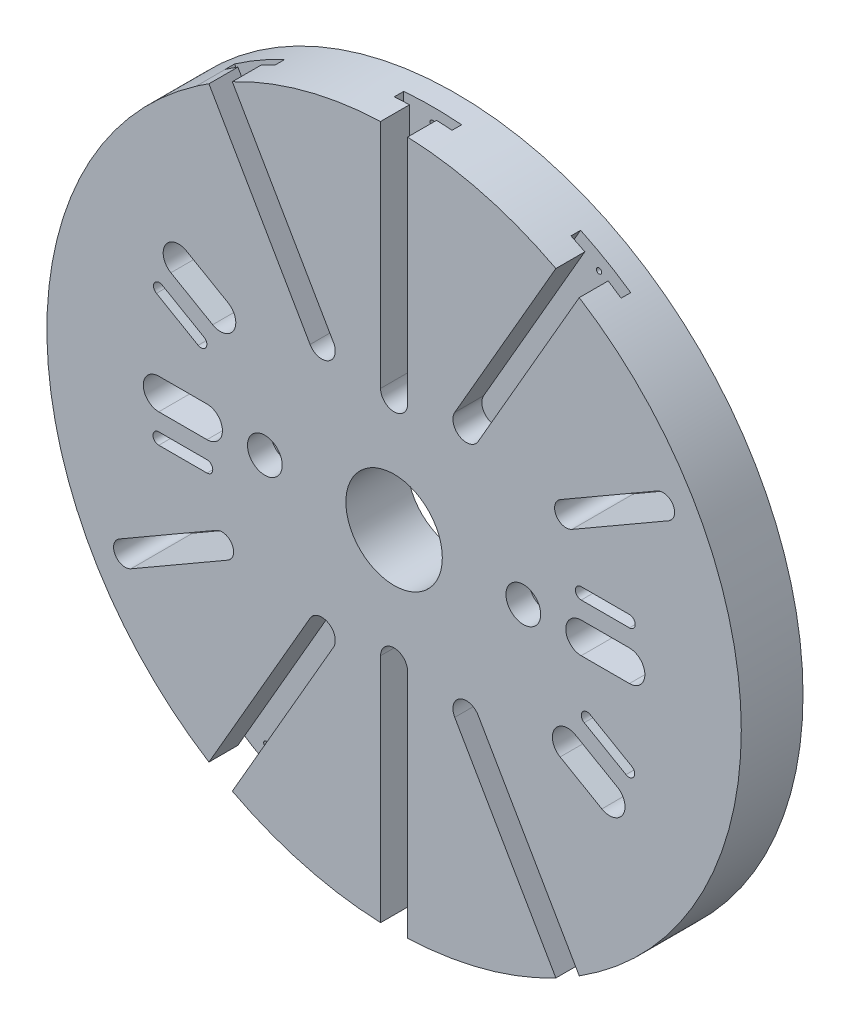
from build123d import *

# Parameters (mm, degrees)
SKETCH1_R           = 180
SKETCH1_R_2         = 25
BOSS_EXTRUDE1_DEPTH = 32
SKETCH2_R           = 5.5
CUT_EXTRUDE1_DEPTH  = 257.561883373
CUT_EXTRUDE3_DEPTH  = 257.561883373
CUT_EXTRUDE4_DEPTH  = 5
CUT_EXTRUDE5_REACH  = 258.562
SKETCH7_R           = 1.375
CUT_EXTRUDE6_DEPTH  = 257.561883373
CUT_EXTRUDE7_DEPTH  = 17.2
CUT_EXTRUDE8_START  = -32
CUT_EXTRUDE8_DEPTH  = 15
SKETCH11_R          = 9
CUT_EXTRUDE9_DEPTH  = 12
SKETCH12_R          = 5.5
CUT_EXTRUDE10_DEPTH = 11


with BuildPart() as part:
    # Sketch1 → Boss-Extrude1 (new body)
    with BuildSketch(Plane.XY):
        Circle(SKETCH1_R)
        Circle(SKETCH1_R_2, mode=Mode.SUBTRACT)
    extrude(amount=BOSS_EXTRUDE1_DEPTH)

    # Sketch2 → Cut-Extrude1 (cut, through all)
    with BuildSketch(Plane.XY.offset(32)):
        with Locations((67, 0)):
            Circle(SKETCH2_R)
        with Locations(Location((-67, 0, 0), (0, 0, 180))):
            Circle(SKETCH2_R)
    extrude(amount=-CUT_EXTRUDE1_DEPTH, mode=Mode.SUBTRACT)

    # Sketch3 → Cut-Extrude3 (cut, through all)
    with BuildSketch(Plane.XY.offset(32)):
        with BuildLine():
            Line((-86.20061659, -56.696152423), (-136.430090009, -85.696152423))
            ThreePointArc((-136.430090009, -85.696152423), (-144.626242432, -83.5), (-142.430090009, -75.303847577))
            Line((-142.430090009, -75.303847577), (-92.20061659, -46.303847577))
            ThreePointArc((-92.20061659, -46.303847577), (-84.004464167, -48.5), (-86.20061659, -56.696152423))
        make_face()
        with BuildLine():
            Line((86.20061659, 56.696152423), (136.430090009, 85.696152423))
            ThreePointArc((136.430090009, 85.696152423), (144.626242432, 83.5), (142.430090009, 75.303847577))
            Line((142.430090009, 75.303847577), (92.20061659, 46.303847577))
            ThreePointArc((92.20061659, 46.303847577), (84.004464167, 48.5), (86.20061659, 56.696152423))
        make_face()
    extrude(amount=-CUT_EXTRUDE3_DEPTH, mode=Mode.SUBTRACT)

    # Sketch5 → Cut-Extrude4 (cut)
    with BuildSketch(Plane(origin=(0, 0, 12), x_dir=(-1, 0, 0), z_dir=(0, 0, -1))):
        with BuildLine():
            Line((15, 60), (15, 264.061054266))
            Line((15, 264.061054266), (-15, 249.37568409))
            Line((-15, 249.37568409), (-15, 60))
            ThreePointArc((-15, 60), (0, 45), (15, 60))
        make_face()
        with BuildLine():
            Line((-91.956389003, 189.273137833), (-117.937151116, 174.273137833))
            Line((-117.937151116, 174.273137833), (-50.490381057, 57.451905284))
            ThreePointArc((-50.490381057, 57.451905284), (-30, 51.961524227), (-24.509618943, 72.451905284))
            Line((-24.509618943, 72.451905284), (-91.956389003, 189.273137833))
        make_face()
        with BuildLine():
            Line((91.956389003, 189.273137833), (24.509618943, 72.451905284))
            ThreePointArc((24.509618943, 72.451905284), (30, 51.961524227), (50.490381057, 57.451905284))
            Line((50.490381057, 57.451905284), (117.937151116, 174.273137833))
            Line((117.937151116, 174.273137833), (91.956389003, 189.273137833))
        make_face()
        with BuildLine():
            Line((91.956389003, -189.273137833), (117.937151116, -174.273137833))
            Line((117.937151116, -174.273137833), (50.490381057, -57.451905284))
            ThreePointArc((50.490381057, -57.451905284), (30, -51.961524227), (24.509618943, -72.451905284))
            Line((24.509618943, -72.451905284), (91.956389003, -189.273137833))
        make_face()
        with BuildLine():
            Line((-91.956389003, -189.273137833), (-24.509618943, -72.451905284))
            ThreePointArc((-24.509618943, -72.451905284), (-30, -51.961524227), (-50.490381057, -57.451905284))
            Line((-50.490381057, -57.451905284), (-117.937151116, -174.273137833))
            Line((-117.937151116, -174.273137833), (-91.956389003, -189.273137833))
        make_face()
        with BuildLine():
            Line((10, -264.061054266), (-15, -249.37568409))
            Line((-15, -249.37568409), (-15, -60))
            ThreePointArc((-15, -60), (0, -45), (15, -60))
            Line((15, -60), (10, -264.061054266))
        make_face()
    extrude(amount=-CUT_EXTRUDE4_DEPTH, mode=Mode.SUBTRACT)

    # Sketch6 → Cut-Extrude5 (cut, up to next)
    with BuildSketch(Plane.XY.offset(32), mode=Mode.PRIVATE) as cut_extrude5_sk1:
        with BuildLine():
            Line((-95.884592233, -180.076985411), (-108.008947886, -173.076985411))
            Line((-108.008947886, -173.076985411), (-43.562177826, -61.451905284))
            ThreePointArc((-43.562177826, -61.451905284), (-34, -58.889727457), (-31.437822174, -68.451905284))
            Line((-31.437822174, -68.451905284), (-95.884592233, -180.076985411))
        make_face()
    cut_extrude5_tool1 = extrude(cut_extrude5_sk1.sketch, amount=-CUT_EXTRUDE5_REACH, mode=Mode.PRIVATE) & part.part
    # Sketch6 → Cut-Extrude5 (cut, up to next)
    with BuildSketch(Plane.XY.offset(32), mode=Mode.PRIVATE) as cut_extrude5_sk2:
        with BuildLine():
            Line((-7, -254.443680545), (-7, -60))
            ThreePointArc((-7, -60), (0, -53), (7, -60))
            Line((7, -60), (7, -245.63245844))
            Line((7, -245.63245844), (-7, -254.443680545))
        make_face()
    cut_extrude5_tool2 = extrude(cut_extrude5_sk2.sketch, amount=-CUT_EXTRUDE5_REACH, mode=Mode.PRIVATE) & part.part
    # Sketch6 → Cut-Extrude5 (cut, up to next)
    with BuildSketch(Plane.XY.offset(32), mode=Mode.PRIVATE) as cut_extrude5_sk3:
        with BuildLine():
            Line((43.562177826, -61.451905284), (108.008947886, -173.076985411))
            Line((108.008947886, -173.076985411), (95.884592233, -180.076985411))
            Line((95.884592233, -180.076985411), (31.437822174, -68.451905284))
            ThreePointArc((31.437822174, -68.451905284), (34, -58.889727457), (43.562177826, -61.451905284))
        make_face()
    cut_extrude5_tool3 = extrude(cut_extrude5_sk3.sketch, amount=-CUT_EXTRUDE5_REACH, mode=Mode.PRIVATE) & part.part
    # Sketch6 → Cut-Extrude5 (cut, up to next)
    with BuildSketch(Plane.XY.offset(32), mode=Mode.PRIVATE) as cut_extrude5_sk4:
        with BuildLine():
            Line((108.008947886, 173.076985411), (95.884592233, 180.076985411))
            Line((95.884592233, 180.076985411), (31.437822174, 68.451905284))
            ThreePointArc((31.437822174, 68.451905284), (34, 58.889727457), (43.562177826, 61.451905284))
            Line((43.562177826, 61.451905284), (108.008947886, 173.076985411))
        make_face()
    cut_extrude5_tool4 = extrude(cut_extrude5_sk4.sketch, amount=-CUT_EXTRUDE5_REACH, mode=Mode.PRIVATE) & part.part
    # Sketch6 → Cut-Extrude5 (cut, up to next)
    with BuildSketch(Plane.XY.offset(32), mode=Mode.PRIVATE) as cut_extrude5_sk5:
        with BuildLine():
            Line((7, 60), (7, 245.63245844))
            Line((7, 245.63245844), (-7, 254.443680545))
            Line((-7, 254.443680545), (-7, 60))
            ThreePointArc((-7, 60), (0, 53), (7, 60))
        make_face()
    cut_extrude5_tool5 = extrude(cut_extrude5_sk5.sketch, amount=-CUT_EXTRUDE5_REACH, mode=Mode.PRIVATE) & part.part
    # Sketch6 → Cut-Extrude5 (cut, up to next)
    with BuildSketch(Plane.XY.offset(32), mode=Mode.PRIVATE) as cut_extrude5_sk6:
        with BuildLine():
            Line((-31.437822174, 68.451905284), (-95.884592233, 180.076985411))
            Line((-95.884592233, 180.076985411), (-108.008947886, 173.076985411))
            Line((-108.008947886, 173.076985411), (-43.562177826, 61.451905284))
            ThreePointArc((-43.562177826, 61.451905284), (-34, 58.889727457), (-31.437822174, 68.451905284))
        make_face()
    cut_extrude5_tool6 = extrude(cut_extrude5_sk6.sketch, amount=-CUT_EXTRUDE5_REACH, mode=Mode.PRIVATE) & part.part
    add(cut_extrude5_tool1.solids().sort_by_distance((-68.344397, -118.375969, 32))[0], mode=Mode.SUBTRACT)
    add(cut_extrude5_tool2.solids().sort_by_distance((-0.052572, -152.280443, 32))[0], mode=Mode.SUBTRACT)
    add(cut_extrude5_tool3.solids().sort_by_distance((68.344397, -118.375969, 32))[0], mode=Mode.SUBTRACT)
    add(cut_extrude5_tool4.solids().sort_by_distance((68.344397, 118.375969, 32))[0], mode=Mode.SUBTRACT)
    add(cut_extrude5_tool5.solids().sort_by_distance((-0.052572, 152.280443, 32))[0], mode=Mode.SUBTRACT)
    add(cut_extrude5_tool6.solids().sort_by_distance((-68.344397, 118.375969, 32))[0], mode=Mode.SUBTRACT)

    # Sketch7 → Cut-Extrude6 (cut, through all)
    with BuildSketch(Plane.XY.offset(32)):
        with Locations((0, 172.5)):
            Circle(SKETCH7_R)
        with Locations((86.25, 149.389382153)):
            Circle(SKETCH7_R)
        with Locations((86.25, -149.389382153)):
            Circle(SKETCH7_R)
        with Locations((0, -172.5)):
            Circle(SKETCH7_R)
        with Locations((-86.25, -149.389382153)):
            Circle(SKETCH7_R)
        with Locations((-86.25, 149.389382153)):
            Circle(SKETCH7_R)
    extrude(amount=-CUT_EXTRUDE6_DEPTH, mode=Mode.SUBTRACT)

    # Sketch8 → Cut-Extrude7 (cut)
    with BuildSketch(Plane.XY.offset(32)):
        with BuildLine():
            Line((97, 8), (122, 8))
            ThreePointArc((122, 8), (130, 0), (122, -8))
            Line((122, -8), (97, -8))
            ThreePointArc((97, -8), (89, 0), (97, 8))
        make_face()
        with BuildLine():
            Line((97, 23), (122, 23))
            ThreePointArc((122, 23), (125, 20), (122, 17))
            Line((122, 17), (97, 17))
            ThreePointArc((97, 17), (94, 20), (97, 23))
        make_face()
        with BuildLine():
            Line((120.217277088, -49.777568136), (98.566641994, -37.277568136))
            ThreePointArc((98.566641994, -37.277568136), (97.468565782, -33.179491924), (101.566641994, -32.081415713))
            Line((101.566641994, -32.081415713), (123.217277088, -44.581415713))
            ThreePointArc((123.217277088, -44.581415713), (124.3153533, -48.679491924), (120.217277088, -49.777568136))
        make_face()
        with BuildLine():
            Line((-97, 8), (-122, 8))
            ThreePointArc((-122, 8), (-130, 0), (-122, -8))
            Line((-122, -8), (-97, -8))
            ThreePointArc((-97, -8), (-89, 0), (-97, 8))
        make_face()
        with BuildLine():
            Line((-122, -17), (-97, -17))
            ThreePointArc((-97, -17), (-94, -20), (-97, -23))
            Line((-97, -23), (-122, -23))
            ThreePointArc((-122, -23), (-125, -20), (-122, -17))
        make_face()
        with BuildLine():
            Line((86.066641994, -58.92820323), (107.717277088, -71.42820323))
            ThreePointArc((107.717277088, -71.42820323), (118.645480318, -68.5), (115.717277088, -57.57179677))
            Line((115.717277088, -57.57179677), (94.066641994, -45.07179677))
            ThreePointArc((94.066641994, -45.07179677), (83.138438763, -48), (86.066641994, -58.92820323))
        make_face()
        with BuildLine():
            Line((-86.066641994, 58.92820323), (-107.717277088, 71.42820323))
            ThreePointArc((-107.717277088, 71.42820323), (-118.645480318, 68.5), (-115.717277088, 57.57179677))
            Line((-115.717277088, 57.57179677), (-94.066641994, 45.07179677))
            ThreePointArc((-94.066641994, 45.07179677), (-83.138438763, 48), (-86.066641994, 58.92820323))
        make_face()
        with BuildLine():
            Line((-120.217277088, 49.777568136), (-98.566641994, 37.277568136))
            ThreePointArc((-98.566641994, 37.277568136), (-97.468565782, 33.179491924), (-101.566641994, 32.081415713))
            Line((-101.566641994, 32.081415713), (-123.217277088, 44.581415713))
            ThreePointArc((-123.217277088, 44.581415713), (-124.3153533, 48.679491924), (-120.217277088, 49.777568136))
        make_face()
    extrude(amount=-CUT_EXTRUDE7_DEPTH, mode=Mode.SUBTRACT)

    # Sketch9 → Cut-Extrude8 (cut)
    with BuildSketch(Plane.XY.offset(32).offset(CUT_EXTRUDE8_START)):
        with BuildLine():
            Line((-104.217277088, 77.490381057), (-82.566641994, 64.990381057))
            ThreePointArc((-82.566641994, 64.990381057), (-77.076260937, 44.5), (-97.566641994, 39.009618943))
            Line((-97.566641994, 39.009618943), (-119.217277088, 51.509618943))
            ThreePointArc((-119.217277088, 51.509618943), (-124.707658145, 72), (-104.217277088, 77.490381057))
        make_face()
        with BuildLine():
            Line((-122, 15), (-97, 15))
            ThreePointArc((-97, 15), (-82, 0), (-97, -15))
            Line((-97, -15), (-122, -15))
            ThreePointArc((-122, -15), (-137, 0), (-122, 15))
        make_face()
        with BuildLine():
            Line((97, -15), (122, -15))
            ThreePointArc((122, -15), (137, 0), (122, 15))
            Line((122, 15), (97, 15))
            ThreePointArc((97, 15), (82, 0), (97, -15))
        make_face()
        with BuildLine():
            Line((104.217277088, -77.490381057), (82.566641994, -64.990381057))
            ThreePointArc((82.566641994, -64.990381057), (77.076260937, -44.5), (97.566641994, -39.009618943))
            Line((97.566641994, -39.009618943), (119.217277088, -51.509618943))
            ThreePointArc((119.217277088, -51.509618943), (124.707658145, -72), (104.217277088, -77.490381057))
        make_face()
    extrude(amount=CUT_EXTRUDE8_DEPTH, mode=Mode.SUBTRACT)

    # Sketch11 → Cut-Extrude9 (cut)
    with BuildSketch(Plane.XY.offset(32)):
        with Locations((-67, 0)):
            Circle(SKETCH11_R)
        with Locations((67, 0)):
            Circle(SKETCH11_R)
    extrude(amount=-CUT_EXTRUDE9_DEPTH, mode=Mode.SUBTRACT)

    # Sketch12 → Cut-Extrude10 (cut)
    with BuildSketch(Plane(origin=(0, 0, 0), x_dir=(-1, 0, 0), z_dir=(0, 0, -1))):
        with Locations((-33.5, -58.023702054)):
            Circle(SKETCH12_R)
        with Locations(Location((33.5, 58.023702054, 0), (0, 0, 180))):
            Circle(SKETCH12_R)
    extrude(amount=-CUT_EXTRUDE10_DEPTH, mode=Mode.SUBTRACT)


solid = part.part
